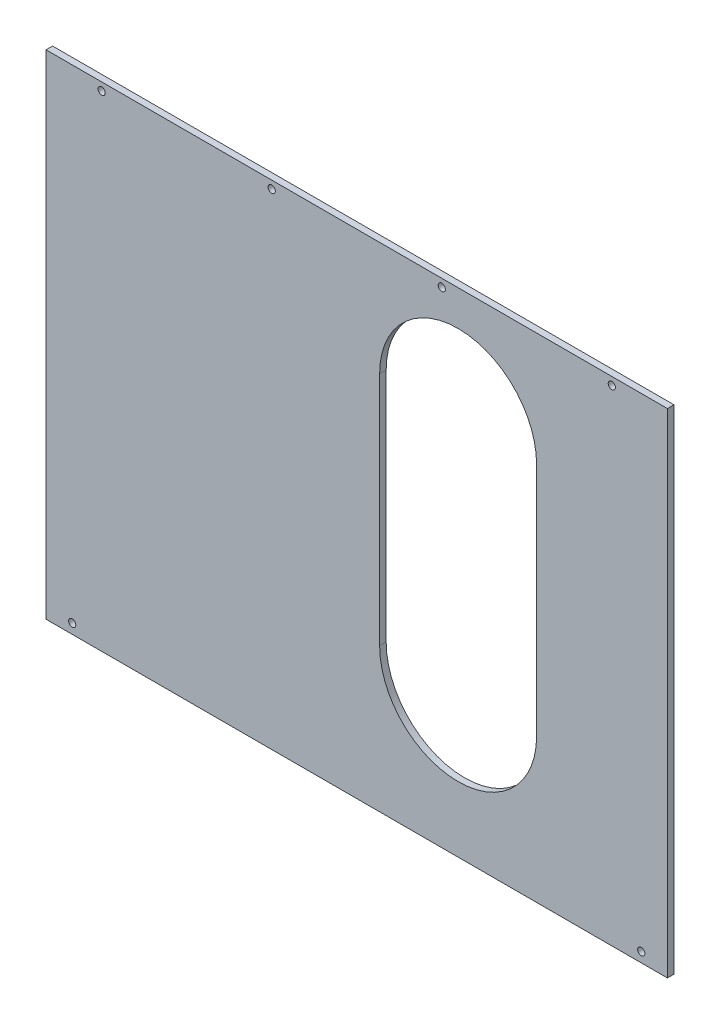
from build123d import *

# Parameters (mm, degrees)
SKETCH1_W            = 475
SKETCH1_H            = 377
BOSS_EXTRUDE1_DEPTH  = 5
M5_CLEARANCE_HOLE1_D = 5.5
CUT_EXTRUDE1_DEPTH   = 10


with BuildPart() as part:
    # Sketch1 → Boss-Extrude1 (new body)
    with BuildSketch(Plane.XY):
        Rectangle(SKETCH1_W, SKETCH1_H)
    extrude(amount=BOSS_EXTRUDE1_DEPTH)

    # M5 Clearance Hole1 (through all)
    with Locations(Plane(origin=(0, 0, 0), x_dir=(-1, 0, 0), z_dir=(0, 0, -1))):
        with Locations((-195, 182.5), (-65, 182.5), (65, 182.5), (195, 182.5), (217.5, -181), (-217.5, -181)):
            Hole(M5_CLEARANCE_HOLE1_D / 2)

    # Sketch3 → Cut-Extrude1 (cut)
    with BuildSketch(Plane(origin=(0, 0, 0), x_dir=(-1, 0, 0), z_dir=(0, 0, -1))):
        with BuildLine():
            Line((-17.5, 101.5), (-17.5, -78.5))
            ThreePointArc((-17.5, -78.5), (-77.5, -138.5), (-137.5, -78.5))
            Line((-137.5, -78.5), (-137.5, 101.5))
            ThreePointArc((-137.5, 101.5), (-77.5, 161.5), (-17.5, 101.5))
        make_face()
    extrude(amount=-CUT_EXTRUDE1_DEPTH, mode=Mode.SUBTRACT)


solid = part.part
